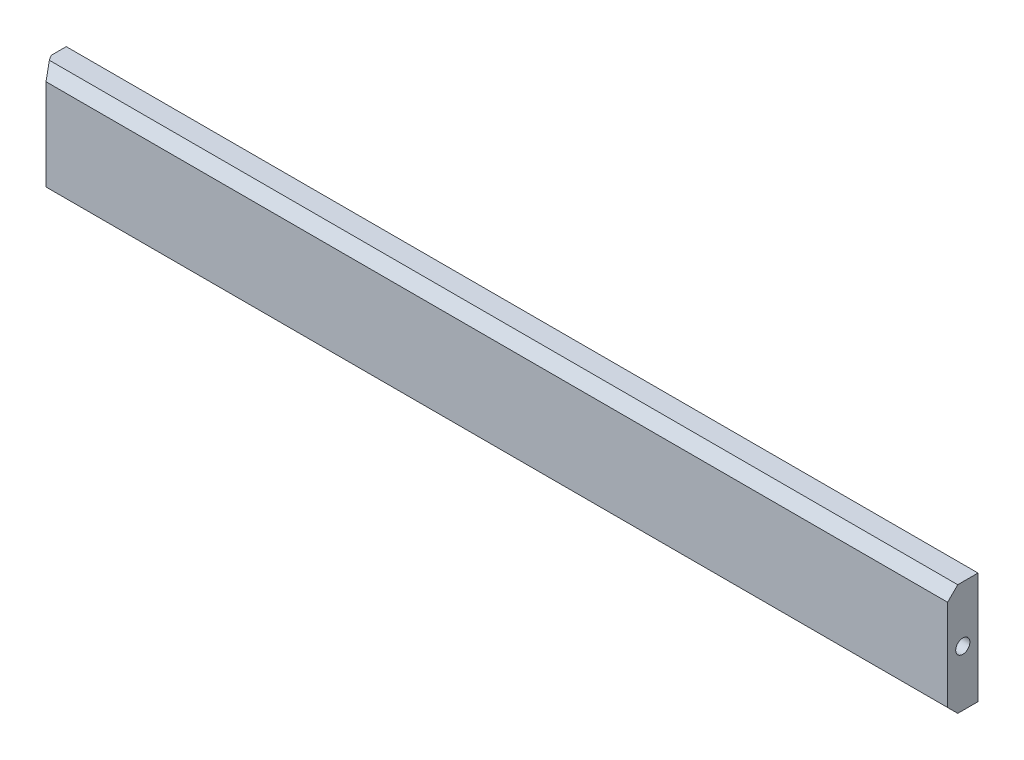
SolidWorks part; units mm, degrees
material "Q235"
ref_plane "Front Plane" through (0, 0, 0) normal (0, 0, 1) x (1, 0, 0)
ref_plane "Top Plane" through (0, 0, 0) normal (0, 1, 0) x (1, 0, 0)
ref_plane "Right Plane" through (0, 0, 0) normal (1, 0, 0) x (0, 0, -1)
sketch "Sketch1" plane through (0, 0, 0) normal (0, 0, 1) x (1, 0, 0)
  line L1 (0, 0) -> (900, 0)
  line L2 (0, 0) -> (0, 110)
  line L3 (0, 110) -> (900, 110)
  line L4 (900, 0) -> (900, 110)
  dimension "D1" = 900
  dimension "D2" = 110
extrude "Boss-Extrude1" add sketch "Sketch1" along normal blind 30
chamfer "Chamfer1" distance 10 angle 45 2 edges at (450, 0, 30) (450, 110, 30)
chamfer "Chamfer2" distance 15 distance2 10 1 edges at (0, 55, 30)
hole_wizard "M16 Tapped Hole1" positions "3DSketch1" profile "Sketch2" tap size "M16" standard "GB"
sketch3d "3DSketch1"
  line L0 (900, 0, 20) -> (900, 0, 0) construction
  line L1 (900, 0, 0) -> (900, 110, 0) construction
  point P0 (900, 55, 15)
  dimension "D1" = 55
  dimension "D2" = 15
sketch "Sketch2" plane through (900, 55, 15) normal (0, 1, 0) x (0, 0, -1)
  line L0 (0, 0) -> (0, 49.206)
  line L1 (0, 49.206) -> (7, 45)
  line L2 (7, 45) -> (7, 0)
  line L5 (7, 0) -> (0, 0)
  line L10 (0, 49.206) -> (-7, 45) construction
  line L11 (0, -6.35) -> (0, 107.95) construction
  dimension "螺纹孔钻头直径" = 14
  dimension "螺纹孔钻头深度" = 45
  dimension "导头角度" = 118
cosmetic thread "Cosmetic thread 1" parameters "D1"=30, "D2"=16
